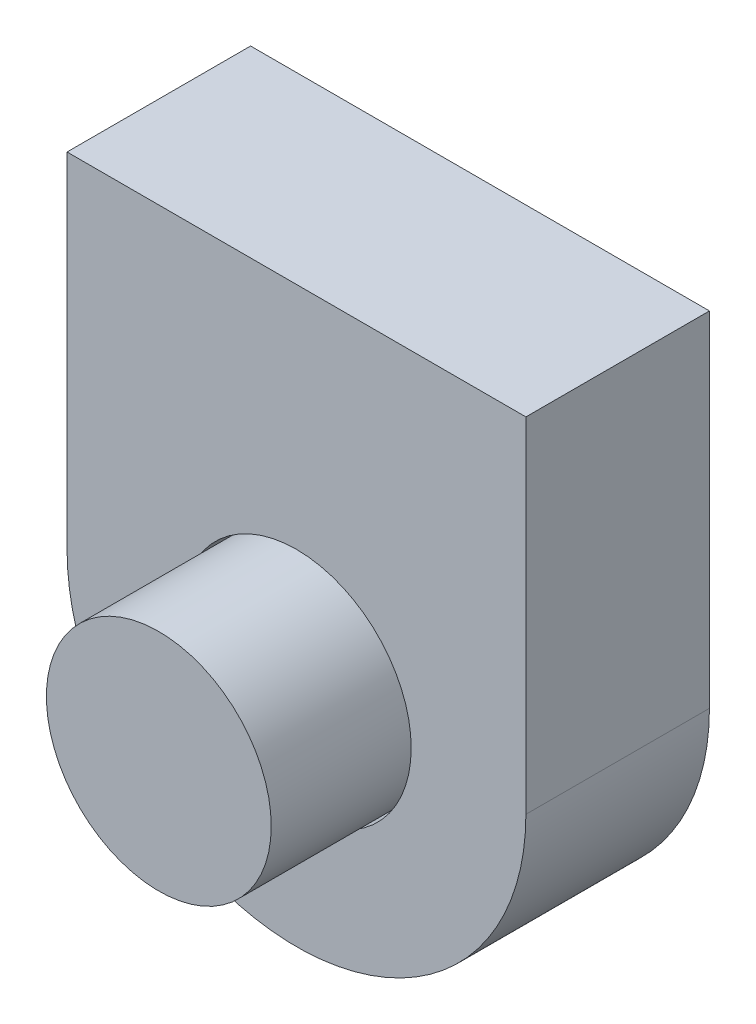
from build123d import *

# Parameters (mm, degrees)
SKETCH3_R           = 5
BOSS_EXTRUDE1_DEPTH = 8
SKETCH6_W           = 4.9
SKETCH6_H           = 14


with BuildPart() as part:
    # Sketch3 → Boss-Extrude1 (new body)
    with BuildSketch(Plane.XY):
        with BuildLine():
            Line((10, 0), (10, 15))
            Line((10, 15), (-10, 15))
            Line((-10, 15), (-10, 0))
            ThreePointArc((-10, 0), (0, -10), (10, 0))
        make_face()
        Circle(SKETCH3_R, mode=Mode.SUBTRACT)
    extrude(amount=-BOSS_EXTRUDE1_DEPTH)


with BuildPart() as body_2:
    # Sketch6 → Revolve2 (revolve)
    with BuildSketch(Plane(origin=(0, 0, 0), x_dir=(1, 0, 0), z_dir=(0, 1, 0))):
        with Locations((2.45, 1)):
            Rectangle(SKETCH6_W, SKETCH6_H)
    revolve(axis=Axis((0, 0, -8), (0, 0, 1)))


solid = Compound([part.part, body_2.part])
